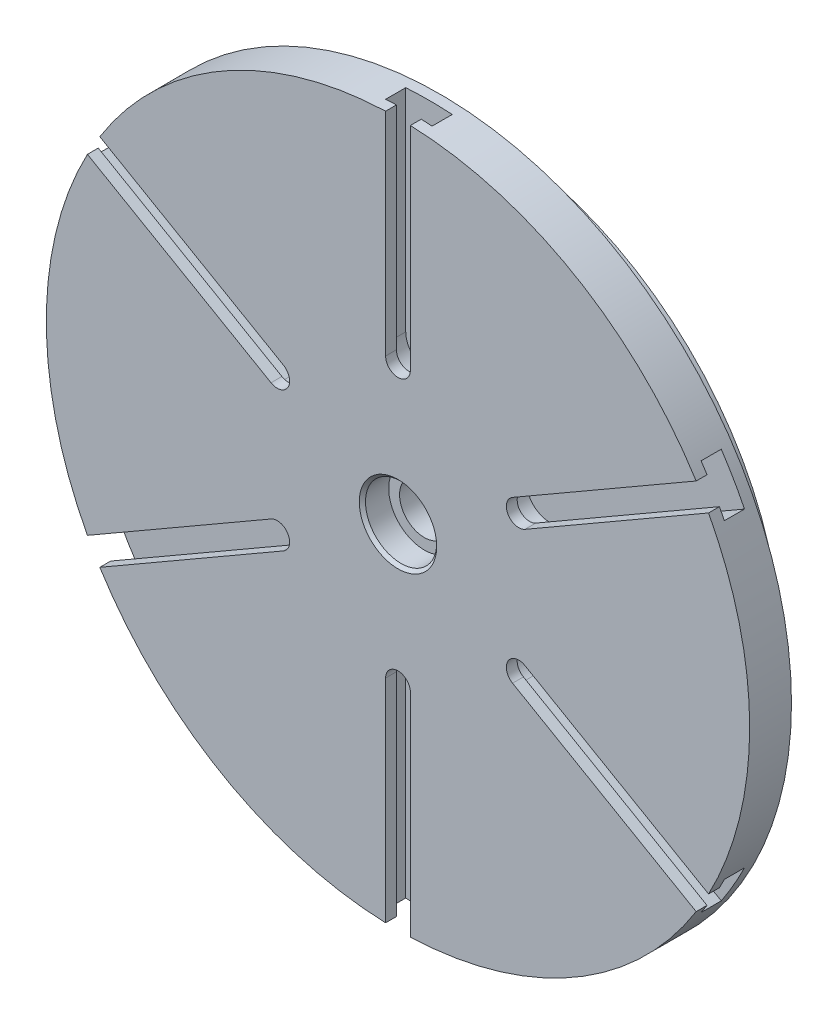
SolidWorks part; units mm, degrees
ref_plane "Front Plane" through (0, 0, 0) normal (0, 0, 1) x (1, 0, 0)
ref_plane "Top Plane" through (0, 0, 0) normal (0, 1, 0) x (1, 0, 0)
ref_plane "Right Plane" through (0, 0, 0) normal (1, 0, 0) x (0, 0, -1)
other "Configuration Table"
sketch "Sketch1" plane through (0, 318.5, 0) normal (0, -1, 0) x (-1, 0, 0)
  line L0 (0, 0) -> (0, 308.6033) construction
  line L1 (176, 77.5) -> (176, 87.5)
  line L2 (176, 87.5) -> (30, 87.5)
  line L3 (30, 87.5) -> (26, 174.5)
  line L4 (-176, 77.5) -> (176, 77.5) construction
  line L5 (176, 77.5) -> (196, 77.5)
  line L6 (196, 77.5) -> (196, 51.1)
  line L7 (196, 51.1) -> (196, 50.1)
  line L8 (196, 50.1) -> (199, 50.1)
  line L9 (199, 50.1) -> (199, 51.1)
  line L10 (199, 51.1) -> (219, 51.1)
  line L11 (219, 51.1) -> (219, 50.1)
  line L12 (219, 50.1) -> (222, 50.1)
  line L13 (26, 174.5) -> (0, 174.5)
  line L14 (222, 50.1) -> (222, 53.1)
  line L15 (222, 53.1) -> (227, 53.1)
  line L16 (227, 53.1) -> (227, 26.1)
  line L17 (0, 174.5) -> (0, 26.1)
  line L18 (227, 26.1) -> (0, 26.1)
  dimension "D1" = 10
  dimension "D2" = 176
  dimension "D3" = 20
  dimension "D4" = 26.4
  dimension "D5" = 3
  dimension "D6" = 1
  dimension "D7" = 26
  dimension "D8" = 3
  dimension "D9" = 2
  dimension "D10" = 5
  dimension "D11" = 27
  dimension "D12" = 30
  dimension "D13" = 87
  dimension "D14" = 26
revolve "Revolve1" add sketch "Sketch1" angle 360 about L0
sketch "Sketch2" plane through (0, 0, -26.1) normal (0, 0, 1) x (1, 0, 0)
  circle A0 centre (0, 318.5) radius 23
  circle A1 centre (0, 318.5) radius 227 construction
  dimension "D1" = 46
extrude "Cut-Extrude1" cut sketch "Sketch2" against normal blind 17
sketch "Sketch3" plane through (0, 0, -43.1) normal (0, 0, 1) x (1, 0, 0)
  circle A0 centre (0, 318.5) radius 16
  dimension "D1" = 32
extrude "Cut-Extrude2" cut sketch "Sketch3" against normal through all
chamfer "Chamfer1" distance 2 angle 45 1 edges at (23, 318.5, -26.1)
sketch "Sketch4" plane through (0, 0, -26.1) normal (0, 0, 1) x (1, 0, 0)
  line L0 (0, 318.5) -> (0, 680.2129) construction
  line L1 (-8, 606.7124) -> (-8, 408.5)
  line L2 (8, 408.5) -> (8, 606.7124)
  line L3 (8, 606.7124) -> (-8, 606.7124)
  arc A0 (-8, 408.5) -> (8, 408.5) centre (0, 408.5) ccw
  dimension "D1" = 8
  dimension "D2" = 90
extrude "Cut-Extrude3" cut sketch "Sketch4" against normal blind 20
ref_plane "Plane1" through (0, 0, -33.1) normal (0, 0, 1) x (1, 0, 0)
sketch "Sketch5" plane through (0, 0, -33.1) normal (0, 0, 1) x (1, 0, 0)
  line L0 (-15, 626.1135) -> (-15, 408.5)
  line L1 (15, 408.5) -> (15, 626.1135)
  line L2 (15, 626.1135) -> (-15, 626.1135)
  arc A0 (-15, 408.5) -> (15, 408.5) centre (0, 408.5) ccw
  arc A1 (-8, 408.5) -> (8, 408.5) centre (0, 408.5) ccw construction
  dimension "D1" = 15
extrude "Cut-Extrude4" cut sketch "Sketch5" against normal blind 13
pattern_circular "CirPattern1" count 6 every 60 about axis through (0, 318.5, 0) along (0, 0, 1) of "Cut-Extrude3", "Cut-Extrude4"
